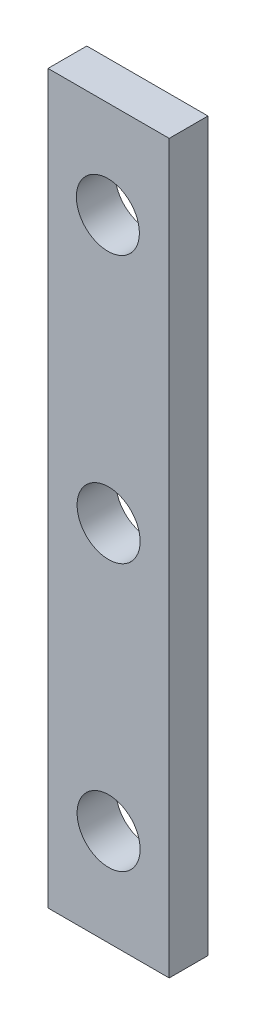
SolidWorks part; units mm, degrees
material "1023 碳钢板 (SS)"
ref_plane "前视基准面" through (0, 0, 0) normal (0, 0, 1) x (1, 0, 0)
ref_plane "上视基准面" through (0, 0, 0) normal (0, 1, 0) x (1, 0, 0)
ref_plane "右视基准面" through (0, 0, 0) normal (1, 0, 0) x (0, 0, -1)
sketch "草图1" plane through (0, 0, 0) normal (0, 0, 1) x (1, 0, 0)
  line L1 (12.5, 75) -> (-12.5, 75)
  line L2 (12.5, 75) -> (12.5, -75)
  line L3 (12.5, -75) -> (-12.5, -75)
  line L4 (-12.5, 75) -> (-12.5, -75)
  line L5 (12.5, 75) -> (-12.5, -75) construction
  line L6 (12.5, -75) -> (-12.5, 75) construction
  circle A0 centre (-0.1539, 54.9998) radius 6.5
  circle A1 centre (0, 0) radius 6.5
  circle A2 centre (0, -55) radius 6.5
  point P0 (0, 0)
  dimension "D3" = 55
  dimension "D4" = 55
  dimension "D5" = 13
  dimension "D1" = 25
  dimension "D2" = 150
extrude "凸台-拉伸1" add sketch "草图1" along normal blind 8
